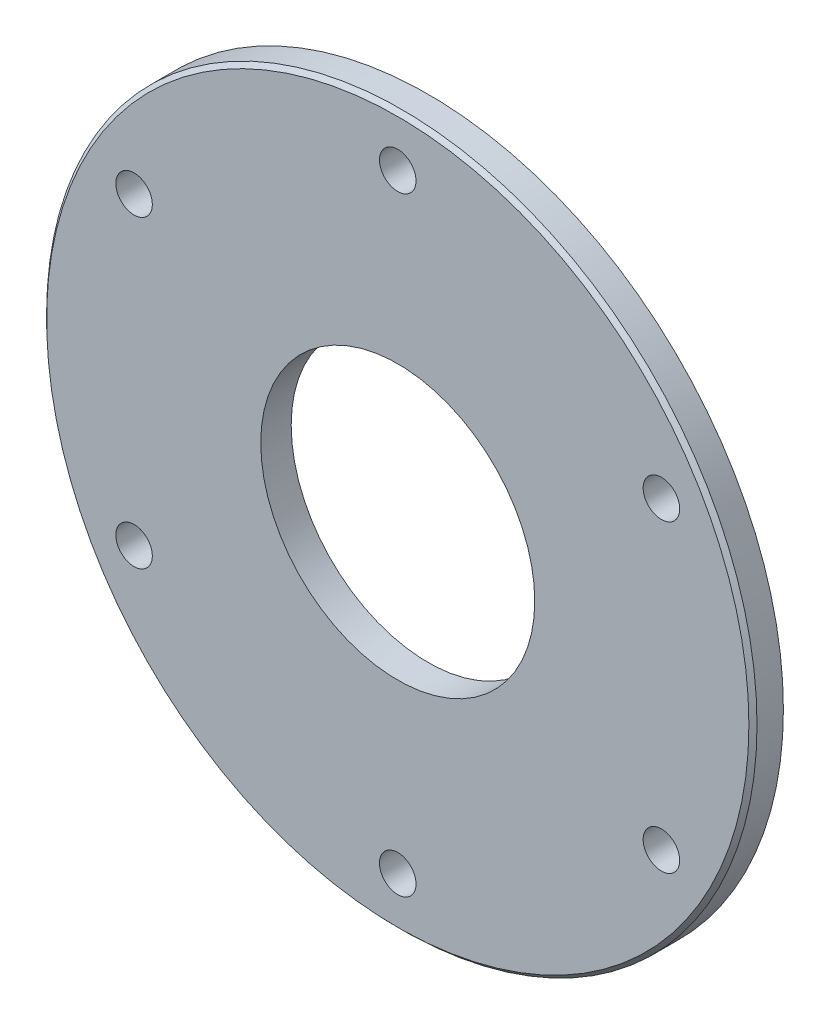
SolidWorks part; units mm, degrees
material "HT200"
ref_plane "Front Plane" through (0, 0, 0) normal (0, 0, 1) x (1, 0, 0)
ref_plane "Top Plane" through (0, 0, 0) normal (0, 1, 0) x (1, 0, 0)
ref_plane "Right Plane" through (0, 0, 0) normal (1, 0, 0) x (0, 0, -1)
sketch "Sketch1" plane through (0, 0, 0) normal (0, 0, 1) x (1, 0, 0)
  circle A0 centre (0, 0) radius 125
  circle A1 centre (0, 0) radius 125 construction
  circle A2 centre (0, 0) radius 110
  dimension "D1" = 15
extrude "Boss-Extrude1" add sketch "Sketch1" along normal up to surface (18 mm away)
sketch "Sketch2" plane through (0, 0, 18) normal (0, 0, 1) x (1, 0, 0)
  circle A0 centre (0, 0) radius 175
  circle A1 centre (0, 150) radius 9
  circle A2 centre (-129.9038, 75) radius 9
  circle A3 centre (-129.9038, -75) radius 9
  circle A4 centre (0, -150) radius 9
  circle A5 centre (129.9038, -75) radius 9
  circle A6 centre (129.9038, 75) radius 9
  arc A7 (140, -105) -> (-140, -105) centre (0, 0) ccw construction
  dimension "D1" = 18
extrude "Boss-Extrude2" add sketch "Sketch2" along normal blind 15
chamfer "Chamfer1" distance 2 angle 45 1 edges at (175, 0, 33)
sketch "Sketch3" plane through (0, 0, 33) normal (0, 0, 1) x (1, 0, 0)
  circle A0 centre (0, 0) radius 67.5
  dimension "D1" = 135
extrude "Cut-Extrude1" cut sketch "Sketch3" against normal through all
